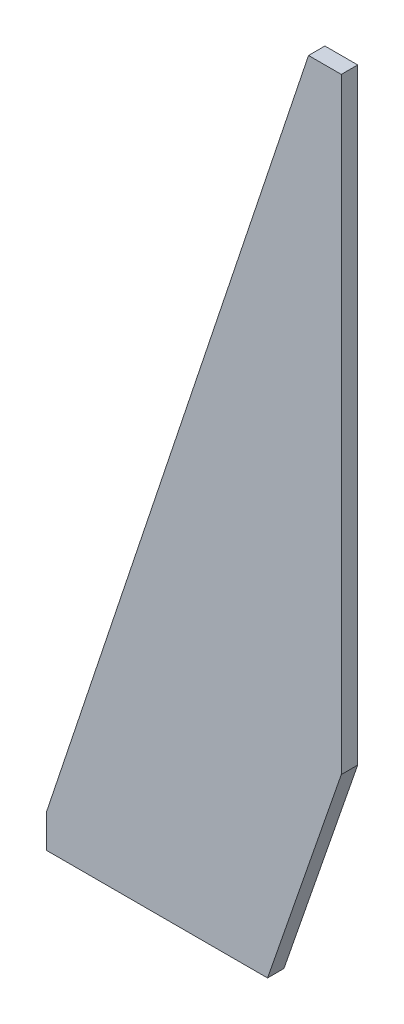
from build123d import *

# Parameters (mm, degrees)
BOSS_EXTRUDE1_DEPTH = 5


with BuildPart() as part:
    # Sketch1 → Boss-Extrude1 (new, symmetric)
    with BuildSketch(Plane.XY):
        Polygon((0, 130), (0, 500), (-20, 500), (-180, 20), (-180, 0), (-45, 0), align=None)
    extrude(amount=BOSS_EXTRUDE1_DEPTH, both=True)


solid = part.part
